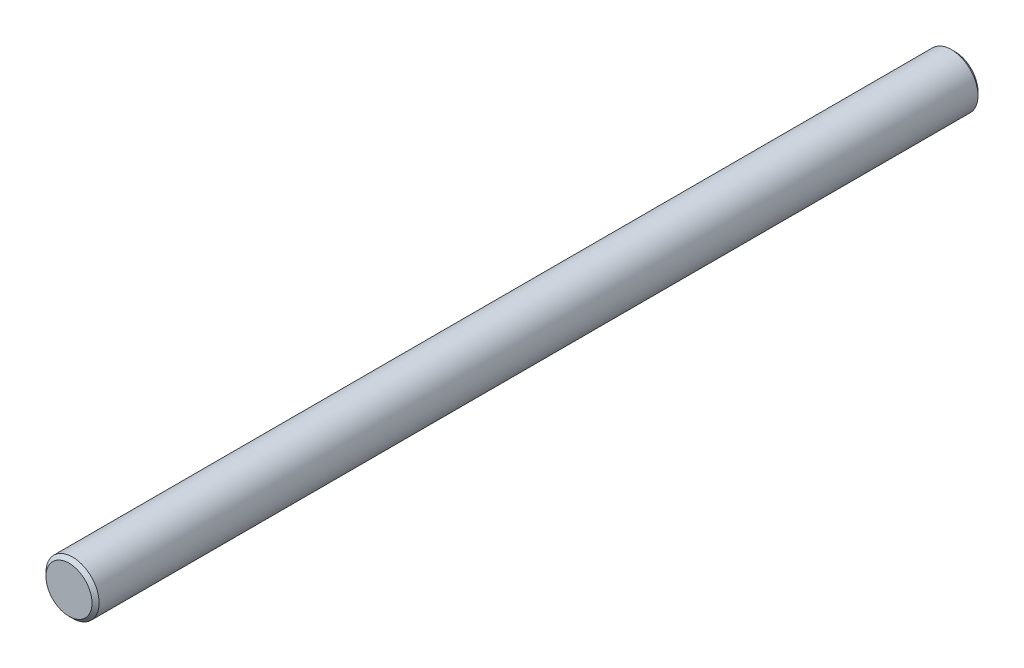
from build123d import *

# Parameters (mm, degrees)
SKETCH1_R           = 1.5
BOSS_EXTRUDE1_DEPTH = 50
SKETCH2_W           = 0.5
SKETCH2_H           = 4
CUT_EXTRUDE1_DEPTH  = 15
CHAMFER1_SIZE       = 0.2


with BuildPart() as part:
    # Sketch1 → Boss-Extrude1 (new body)
    with BuildSketch(Plane.XY):
        Circle(SKETCH1_R)
    extrude(amount=BOSS_EXTRUDE1_DEPTH)

    # Sketch2 → Cut-Extrude1 (cut, symmetric)
    with BuildSketch(Plane(origin=(0, 0, 0), x_dir=(1, 0, 0), z_dir=(0, 1, 0))):
        with Locations((-1.25, -4)):
            Rectangle(SKETCH2_W, SKETCH2_H)
    extrude(amount=CUT_EXTRUDE1_DEPTH, both=True, mode=Mode.SUBTRACT)

    # Chamfer1
    chamfer1_edges = [part.edges().sort_by_distance(p)[0] for p in [
        (-1.5, 0, 0),
        (-1.5, 0, 50),
    ]]
    chamfer(chamfer1_edges, length=CHAMFER1_SIZE)


solid = part.part
